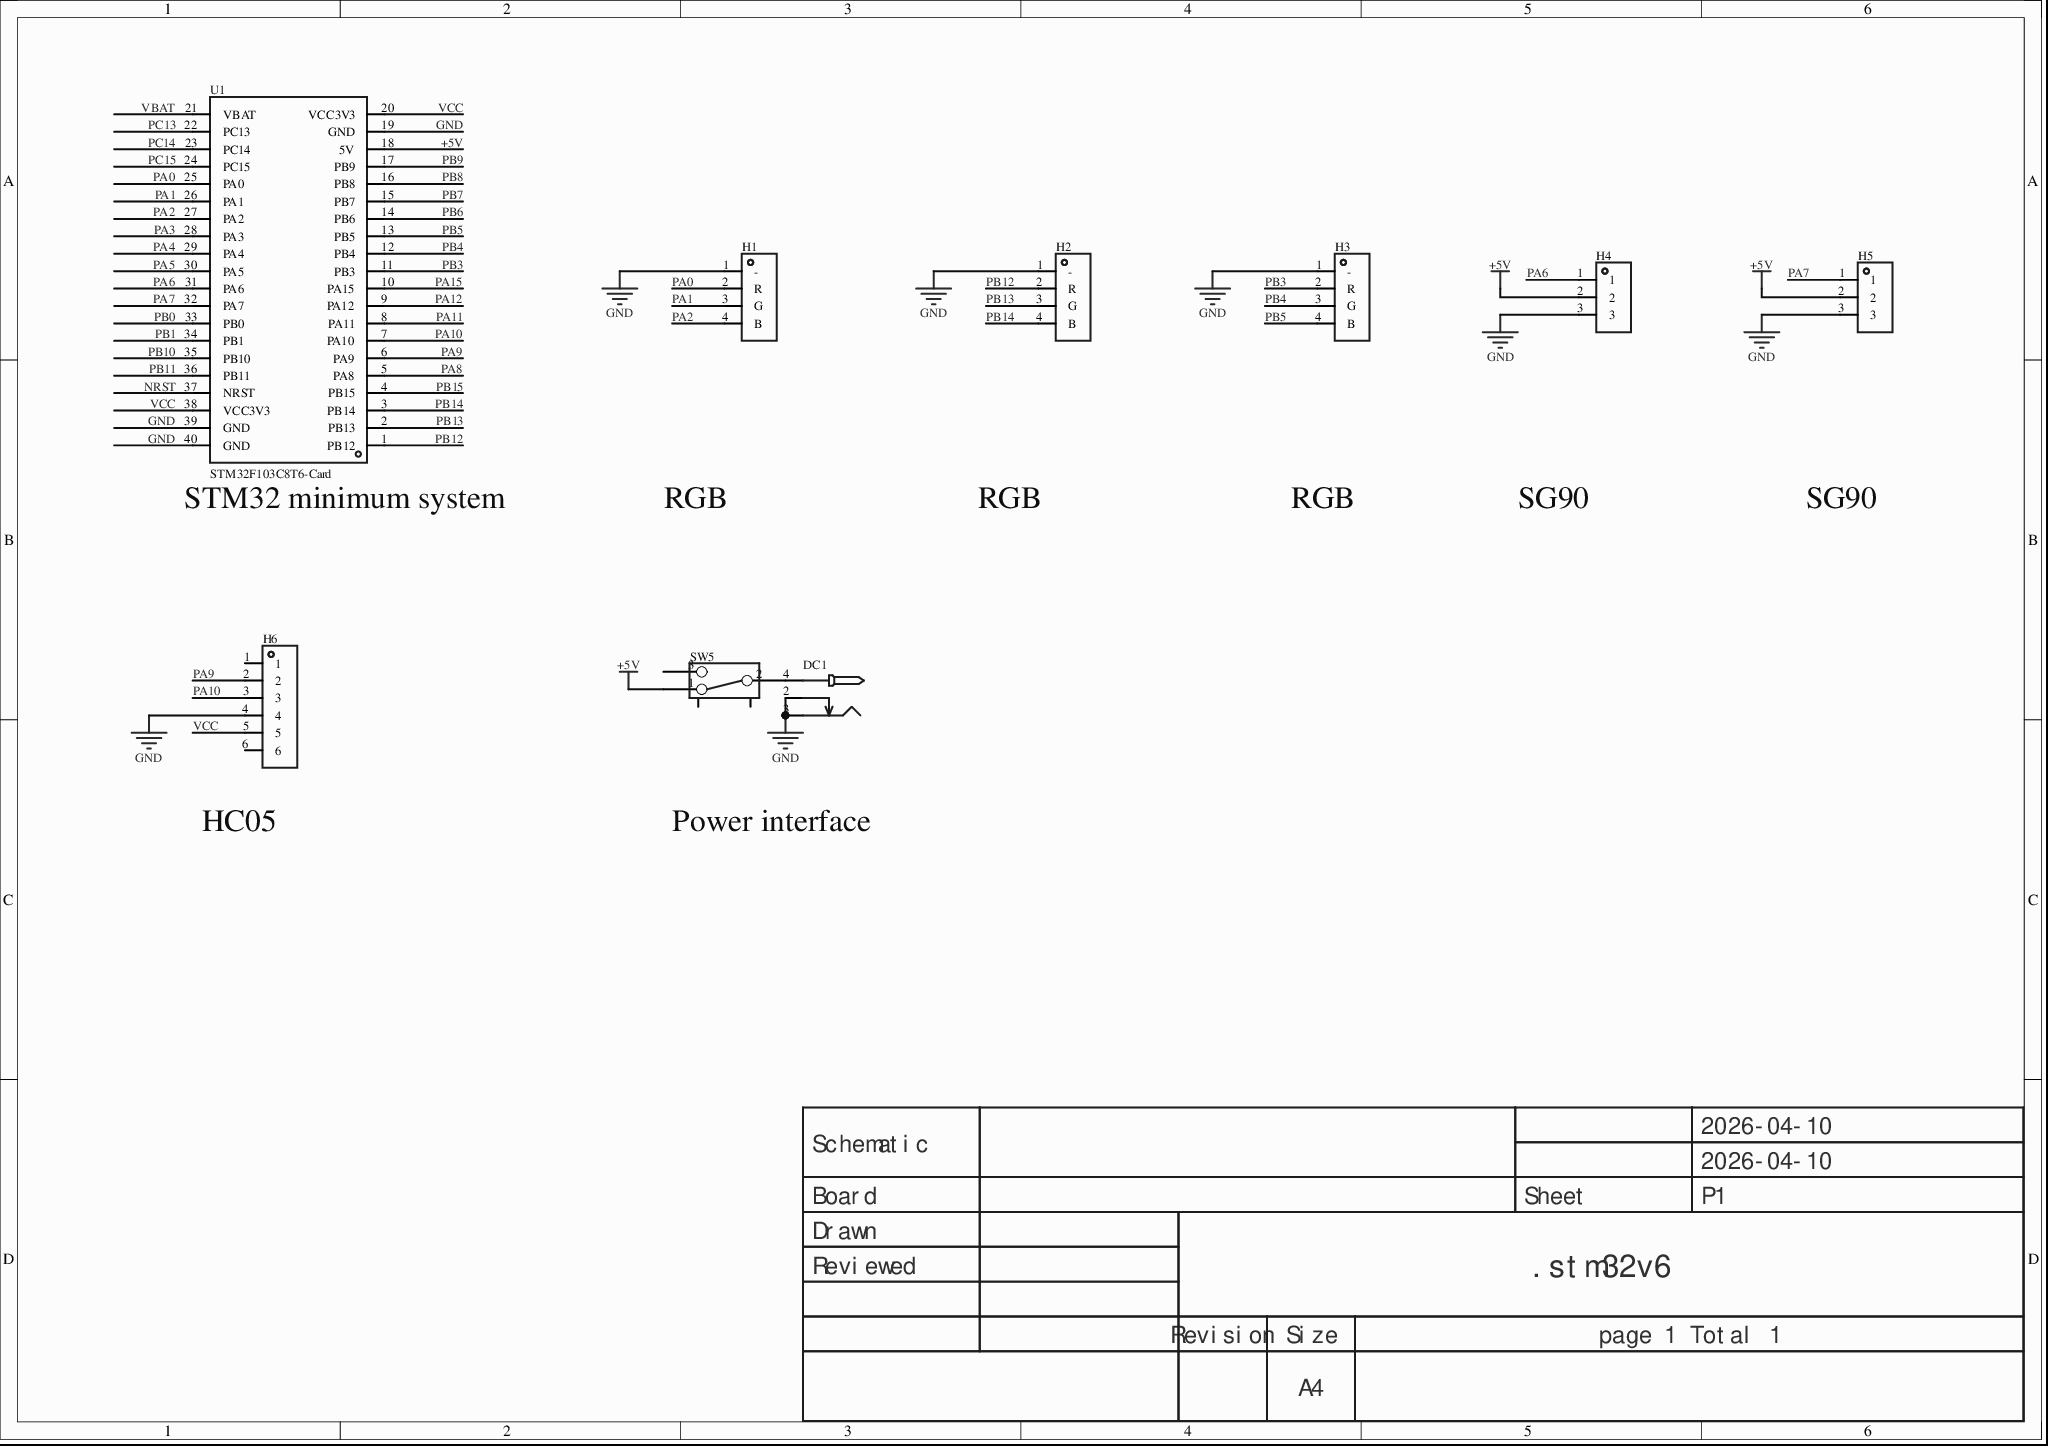
[diagram p0: MISC51537-3.schdoc]
# Altium project MISC51537-2.PrjPcb
1 sheet, 9 parts. Net scope: global (net labels, ports and power ports of the same name join across sheets).
Board file: MISC51537.pcbdoc

## Sheet MISC51537-3.schdoc
size 297 x 209 mm; Version: V1.0; @Project Name: MISC51537; @Page Count: 1; @Update Date: 2026-04-10; @Create Date: 2026-04-10; @Schematic Name: MISC51537; @Page No: 1; @Create Time: 23:22:16; @Update Time: 17:32:40; @Board Name: MISC51537

### Parts
DC1  (no value)  [DC-2.0]
H1  (no value)  [HDR-TH_4P-P2.54-V-F]
H2  (no value)  [HDR-TH_4P-P2.54-V-F]
H3  (no value)  [HDR-TH_4P-P2.54-V-F]
H4  (no value)  [HDR-TH_3P-P2.54-V-M]
H5  (no value)  [HDR-TH_3P-P2.54-V-M]
H6  (no value)  [HDR-TH_6P-P2.54-V-F]
SW5  (no value)  [拨动开关]
U1  STM32F103C8T6-Card  [CONN-TH_L53.3-W22.9_STM32F103C8T6-CARD]

### Nets
+5V: H4.2 H5.2 SW5.1 U1.18(5V)
GND: DC1.2 DC1.3 H1.1(-) H2.1(-) H3.1(-) H4.3 H5.3 H6.4 U1.19(GND) U1.39(GND) U1.40(GND)
VCC: H6.5 U1.20(VCC3V3) U1.38(VCC3V3)
NRST: U1.37(NRST)
PA0: H1.2(R) U1.25(PA0)
PA1: H1.3(G) U1.26(PA1)
PA2: H1.4(B) U1.27(PA2)
PA3: U1.28(PA3)
PA4: U1.29(PA4)
PA5: U1.30(PA5)
PA6: H4.1 U1.31(PA6)
PA7: H5.1 U1.32(PA7)
PA8: U1.5(PA8)
PA9: H6.2 U1.6(PA9)
PA10: H6.3 U1.7(PA10)
PA11: U1.8(PA11)
PA12: U1.9(PA12)
PA15: U1.10(PA15)
PB0: U1.33(PB0)
PB1: U1.34(PB1)
PB3: H3.2(R) U1.11(PB3)
PB4: H3.3(G) U1.12(PB4)
PB5: H3.4(B) U1.13(PB5)
PB6: U1.14(PB6)
PB7: U1.15(PB7)
PB8: U1.16(PB8)
PB9: U1.17(PB9)
PB10: U1.35(PB10)
PB11: U1.36(PB11)
PB12: H2.2(R) U1.1(PB12)
PB13: H2.3(G) U1.2(PB13)
PB14: H2.4(B) U1.3(PB14)
PB15: U1.4(PB15)
PC13: U1.22(PC13)
PC14: U1.23(PC14)
PC15: U1.24(PC15)
VBAT: U1.21(VBAT)
NetDC1_4: DC1.4 SW5.2

Not connected (* = marked no-connect by the designer): H6 1 6; SW5 3 4 5

### Notes on the sheet
- (near U1) STM32 minimum system
- RGB
- SG90
- (near H6) HC05
- Power interface
- Labels drawn without touching a wire or pin: VCC
- 2026-04-10
- Schematic
- Board
- Sheet
- P1
- Drawn
- Reviewed
- .stm32v6
- Revision
- Size
- A4
- page 1 Total 1

### Library data of the parts
DC1 = DC-005_2.0: Symbol: DC power jack; ConvertToPcb: yes; ModelId: f5f20b8a2308479b936ba3c2698865bb0819f05c4eef4c71ace90d822a990e87; ModelName: DC-IN-TH_DC-5520-1; ModelTransform: 372.05,551.18,582.68,90,0,0,137.8,0,-149.61; Device: DC-005_2.0; AddInBom: yes; Supplier Footprint: 插件; FootprintName: DC-2.0
H1-H3 = HDR-F_2.54_1x4P: Symbol: 2.54-1*4P female; ConvertToPcb: yes; ModelId: d187812051054f85879fcaa51a310d8e0819f05c4eef4c71ace90d822a990e87; ModelTransform: 419.6842,98.464,0,0,0,0,0,0,-118.11; Device: HDR-F_2.54_1x4P; AddInBom: yes; SupplierPart: C2718488; Supplier Footprint: 插件; FootprintName: HDR-TH_4P-P2.54-V-F; ModelName: HDR-TH_4P-P2.54-V-F
H4 H5 = HDR-M_2.54_1x3P: AddInBom: yes; ModelId: bb473b6d38ff42a99216a4fcdbdcc4cb0819f05c4eef4c71ace90d822a990e87; ModelName: HDR-TH_3P-P2.54-M-LI-1X3P; ModelTransform: 300.03877,100,0,0,0,0,0,0,-118.11; Symbol: HDR-M_2.54_1x3P; Device: HDR-M_2.54_1x3P; ConvertToPcb: yes; FootprintName: HDR-TH_3P-P2.54-V-M; SupplierPart: C2937625; Supplier Footprint: 插件
H6 = HDR-F_2.54_1x6P: Symbol: Header-Female-2.54_1x6; ConvertToPcb: yes; ModelId: 0f5bcf94dcda47d085f24cdca1696fe9; ModelTransform: 619.684,94.488,0,0,0,0,0,0,-125.984; Device: HDR-F_2.54_1x6P; AddInBom: yes; SupplierPart: C40877; Supplier Footprint: 插件; FootprintName: HDR-TH_6P-P2.54-V-F; ModelName: HDR-TH_6P-P2.54-V-F
SW5 = 拨动开关_正: Symbol: Toggle switch; Device: Toggle switch (positive); ConvertToPcb: yes; ModelId: 4321fe59a4074cbfb4989553f297c68f0819f05c4eef4c71ace90d822a990e87; ModelName: SW-TH_SS-12D02-VG4; ModelTransform: 370.09,208.7,472.35,0,0,0,0,0,-110; AddInBom: yes; Supplier Footprint: 插件; FootprintName: Toggle switch
U1 = STM32F103C8T6-Card: AddInBom: yes; Symbol: STM32F103C8T6-CARD; Device: STM32F103C8T6-Card; LCSC Part Name: STM32F103C8T6-Card; SupplierPart: C9900077949; ManufacturerPart: STM32F103C8T6-Card; Supplier Footprint: 插件; Supplier: LCSC; ConvertToPcb: yes; FootprintName: CONN-TH_L53.3-W22.9_STM32F103C8T6-CARD